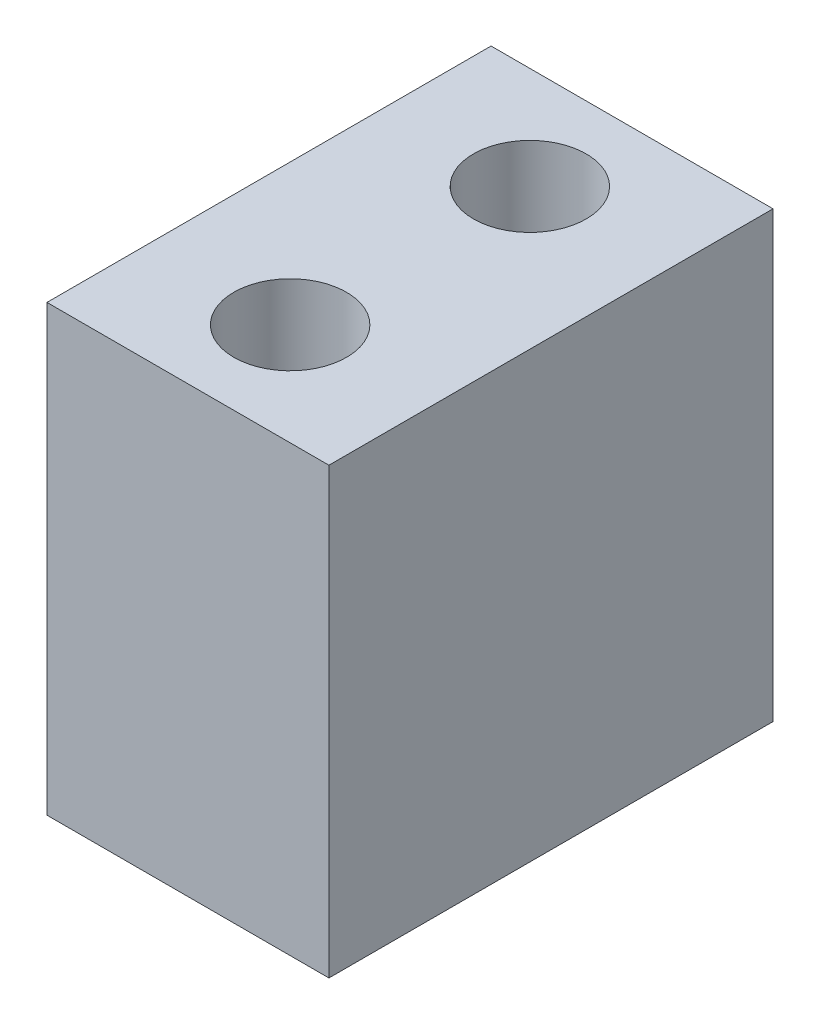
SolidWorks part; units mm, degrees
material "Q235"
ref_plane "Front Plane" through (0, 0, 0) normal (0, 0, 1) x (1, 0, 0)
ref_plane "Top Plane" through (0, 0, 0) normal (0, 1, 0) x (1, 0, 0)
ref_plane "Right Plane" through (0, 0, 0) normal (1, 0, 0) x (0, 0, -1)
sketch "Sketch2" plane through (0, 0, 0) normal (0, 1, 0) x (1, 0, 0)
  line L0 (-131.395, 0) -> (113.7022, 0) construction
  line L1 (0, 164.1787) -> (0, -121.5078) construction
  line L3 (-40, 63) -> (40, 63)
  line L4 (-40, 63) -> (-40, -63)
  line L5 (-40, -63) -> (40, -63)
  line L6 (40, 63) -> (40, -63)
  dimension "D1" = 126
  dimension "D2" = 80
  dimension "D3" = 40
extrude "Boss-Extrude1" add sketch "Sketch2" along normal mid plane 126
hole_wizard "M36 Tapped Hole1" positions "Sketch4" profile "Sketch3" tap size "M36" standard "GB"
sketch "Sketch4" plane through (0, 63, 0) normal (0, 1, 0) x (1, 0, 0)
  line L0 (0, 87.994) -> (0, -83.4139) construction
  line L2 (-50.2782, 0) -> (51.8371, 0) construction
  point P0 (0, 34)
  point P3 (0, -34)
  dimension "D1" = 68
cosmetic thread "Cosmetic Thread1"
cosmetic thread "Cosmetic Thread2"
sketch "Sketch3" plane through (0, 63, -34) normal (1, 0, 0) x (0, 0, 1)
  line L0 (0, 0) -> (0, 89.6138)
  line L1 (0, 89.6138) -> (16, 80)
  line L2 (16, 80) -> (16, 0)
  line L5 (16, 0) -> (0, 0)
  line L10 (0, 89.6138) -> (-16, 80) construction
  line L11 (0, -6.35) -> (0, 107.95) construction
  dimension "螺纹孔钻头直径" = 32
  dimension "螺纹孔钻头深度" = 80
  dimension "导头角度" = 118
